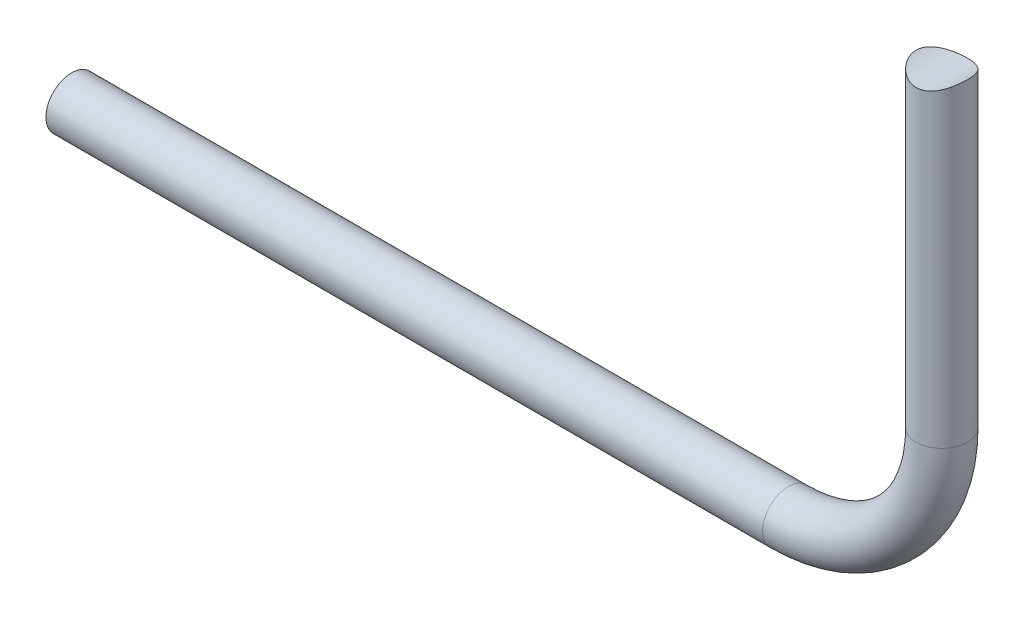
SolidWorks part; units mm, degrees
material "1023 碳钢板 (SS)"
ref_plane "前视基准面" through (0, 0, 0) normal (0, 0, 1) x (1, 0, 0)
ref_plane "上视基准面" through (0, 0, 0) normal (0, 1, 0) x (1, 0, 0)
ref_plane "右视基准面" through (0, 0, 0) normal (1, 0, 0) x (0, 0, -1)
sketch "草图1" plane through (0, 0, 0) normal (0, 0, 1) x (1, 0, 0)
  line L0 (0, 0) -> (140, 0)
  line L1 (170, 30) -> (170, 95)
  arc A0 (140, 0) -> (170, 30) centre (140, 30) ccw
  point P7 (170, 0)
  dimension "D2" = 30
  dimension "D1" = 170
  dimension "D3" = 95
sketch "草图2" plane through (0, 0, 0) normal (1, 0, 0) x (0, 0, -1)
  circle A0 centre (0, 0) radius 5
  dimension "D1" = 10
sweep "扫描1" add profiles "草图2" path "草图1"
sketch "草图3" plane through (0, 0, 0) normal (0, 0, 1) x (1, 0, 0)
  line L0 (0, -5) -> (237.0674, -5) construction
  circle A0 centre (170, 100) radius 10
  dimension "D1" = 20
  dimension "D2" = 105
extrude "切除-拉伸1" cut sketch "草图3" against normal mid plane 10
